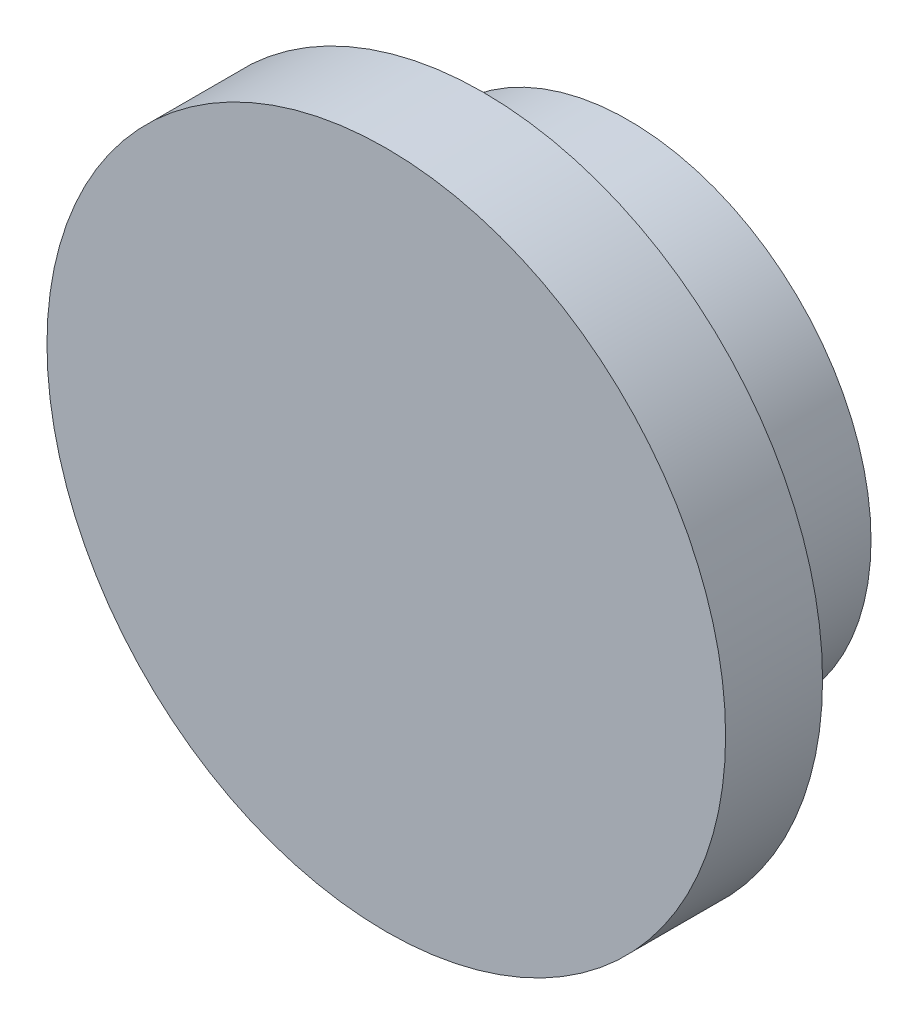
from build123d import *

# Parameters (mm, degrees)
SKETCH_1_R      = 5
EXTRUDE_1_DEPTH = 3
SKETCH_2_R      = 7
EXTRUDE_2_DEPTH = 2


with BuildPart() as part:
    # 草图1 → 凸台-拉伸1 (new body)
    with BuildSketch(Plane.XY):
        Circle(SKETCH_1_R)
    extrude(amount=-EXTRUDE_1_DEPTH)

    # 草图2 → 凸台-拉伸2 (add)
    with BuildSketch(Plane.XY):
        Circle(SKETCH_2_R)
    extrude(amount=EXTRUDE_2_DEPTH)


solid = part.part
